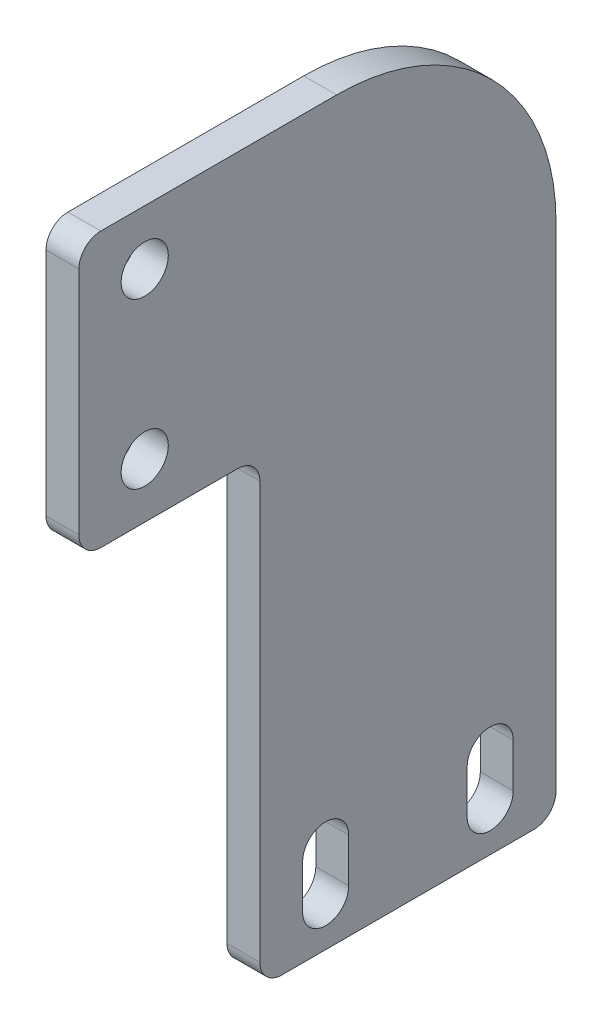
SolidWorks part; units mm, degrees
material "不锈钢201"
ref_plane "前视基准面" through (0, 0, 0) normal (0, 0, 1) x (1, 0, 0)
ref_plane "上视基准面" through (0, 0, 0) normal (0, 1, 0) x (1, 0, 0)
ref_plane "右视基准面" through (0, 0, 0) normal (1, 0, 0) x (0, 0, -1)
sketch "草图1" plane through (0, 0, 0) normal (1, 0, 0) x (0, 0, -1)
  line L0 (0, 33.5) -> (0, -7.9603) construction
  line L1 (-12.5, 6) -> (-6, 6)
  line L2 (-12.5, 6) -> (-12.5, -6)
  line L3 (-12.5, -6) -> (12.5, -6)
  line L4 (12.5, 6) -> (12.5, -6)
  line L5 (-12.5, 6) -> (12.5, -6) construction
  line L6 (-12.5, -6) -> (12.5, 6) construction
  line L7 (-6, 61) -> (6, 61)
  line L8 (-6, 61) -> (-6, 6)
  line L10 (6, 61) -> (6, 6)
  line L11 (-6, 61) -> (6, 6) construction
  line L12 (-6, 6) -> (6, 61) construction
  line L14 (6, 6) -> (12.5, 6)
  point P0 (0, 0)
  point P6 (0, 33.5)
  dimension "D1" = 12
  dimension "D2" = 25
  dimension "D3" = 12
  dimension "D4" = 55
extrude "凸台-拉伸1" add sketch "草图1" along normal blind 3
sketch "草图2" plane through (0, 0, 0) normal (-1, 0, 0) x (0, 0, 1)
  line L0 (-6, 61) -> (-12.5, 6)
  line L1 (6, 61) -> (12.5, 6)
  line L2 (-6, 61) -> (6, 61)
  line L3 (-12.5, 6) -> (12.5, 6)
extrude "凸台-拉伸2" add sketch "草图2" against normal up to surface (3 mm away) up to face at (3, 16.75, 0)
fillet "圆角1" [suppressed] radius 2
sketch "草图3" plane through (0, 0, 0) normal (-1, 0, 0) x (0, 0, 1)
  line L0 (-9.6408, 0) -> (9.298, 0) construction
  line L1 (0, 0) -> (0, -6.9973) construction
  line L2 (-7.5, 2) -> (-7.5, -2) construction
  line L3 (-5.4, 2) -> (-5.4, -2)
  line L4 (-9.6, 2) -> (-9.6, -2)
  line L5 (7.5, 2) -> (7.5, -2) construction
  line L6 (5.4, 2) -> (5.4, -2)
  line L7 (9.6, 2) -> (9.6, -2)
  line L8 (12.5, -6) -> (-12.5, -6) construction
  arc A0 (-5.4, 2) -> (-9.6, 2) centre (-7.5, 2) ccw
  arc A1 (-9.6, -2) -> (-5.4, -2) centre (-7.5, -2) ccw
  arc A2 (5.4, 2) -> (9.6, 2) centre (7.5, 2) cw
  arc A3 (9.6, -2) -> (5.4, -2) centre (7.5, -2) cw
  point P7 (-7.5, 0)
  point P14 (7.5, 0)
  dimension "D4" = 2.1
  dimension "D1" = 15
  dimension "D2" = 4
  dimension "D3" = 6
extrude "切除-拉伸1" cut sketch "草图3" against normal blind 3
fillet "圆角2" radius 2 2 edges at (1.5, -6, -12.5) (1.5, -6, 12.5)
hole_wizard "Ø4.3 (4.3) 直径孔1" positions "草图4" profile "草图6" hole size "Ø4.3" standard "GB"
sketch "草图4" plane through (0, 0, 0) normal (-1, 0, 0) x (0, 0, 1)
  point P0 (0, 56)
  point P3 (0, 41)
sketch "草图6" plane through (0, 56, 0) normal (0, 1, 0) x (0, 0, 1)
  line L0 (0, 0) -> (0, 11.3919)
  line L1 (0, 11.3919) -> (2.15, 10.1)
  line L2 (2.15, 10.1) -> (2.15, 0)
  line L5 (2.15, 0) -> (0, 0)
  line L10 (0, 11.3919) -> (-2.15, 10.1) construction
  line L11 (0, -6.35) -> (0, 107.95) construction
  dimension "孔直径" = 4.3
  dimension "孔深度" = 10.1
  dimension "导头角度" = 118
sketch "草图7" plane through (0, 0, 0) normal (-1, 0, 0) x (0, 0, 1)
  line L0 (-6, 61) -> (6, 61) construction
  line L1 (-3.5669, 61) -> (-37.5, 61)
  line L2 (-3.5669, 61) -> (-3.5669, 36)
  line L3 (-3.5669, 36) -> (-10.5, 36)
  line L4 (-37.5, 61) -> (-37.5, -6)
  line L5 (-10.5, -6) -> (-37.5, -6)
  line L6 (-10.5, -6) -> (-10.5, 36)
  line L7 (-12.5, -4) -> (-12.5, 6) construction
  dimension "D1" = 25
  dimension "D2" = 25
extrude "凸台-拉伸3" add sketch "草图7" against normal up to surface (3 mm away) up to face at (3, 56, -2.15)
pattern_linear "阵列(线性)1" count 2 spacing 24 along (0, 0, -1) of "切除-拉伸1"
sketch "草图8" plane through (0, 0, 0) normal (-1, 0, 0) x (0, 0, 1)
  line L1 (-10.5, 36) -> (13.7212, 36)
  line L2 (-10.5, 36) -> (-10.5, -7.9757)
  line L3 (-10.5, -7.9757) -> (13.7212, -7.9757)
  line L4 (13.7212, 36) -> (13.7212, -7.9757)
extrude "切除-拉伸2" cut sketch "草图8" against normal blind 10
sketch "草图9" plane through (0, 0, 0) normal (-1, 0, 0) x (0, 0, 1)
  line L1 (6, 61) -> (14.5945, 61)
  line L2 (6, 61) -> (6, 31.8446)
  line L3 (6, 31.8446) -> (14.5945, 31.8446)
  line L4 (14.5945, 61) -> (14.5945, 31.8446)
extrude "切除-拉伸3" cut sketch "草图9" against normal blind 10
fillet "圆角3" radius 2 5 edges at (1.5, 36, -10.5) (1.5, 36, 6) (1.5, 61, 6) (1.5, -6, -10.5) (1.5, -6, -37.5)
fillet "圆角4" radius 20 1 edges at (1.5, 61, -37.5)
